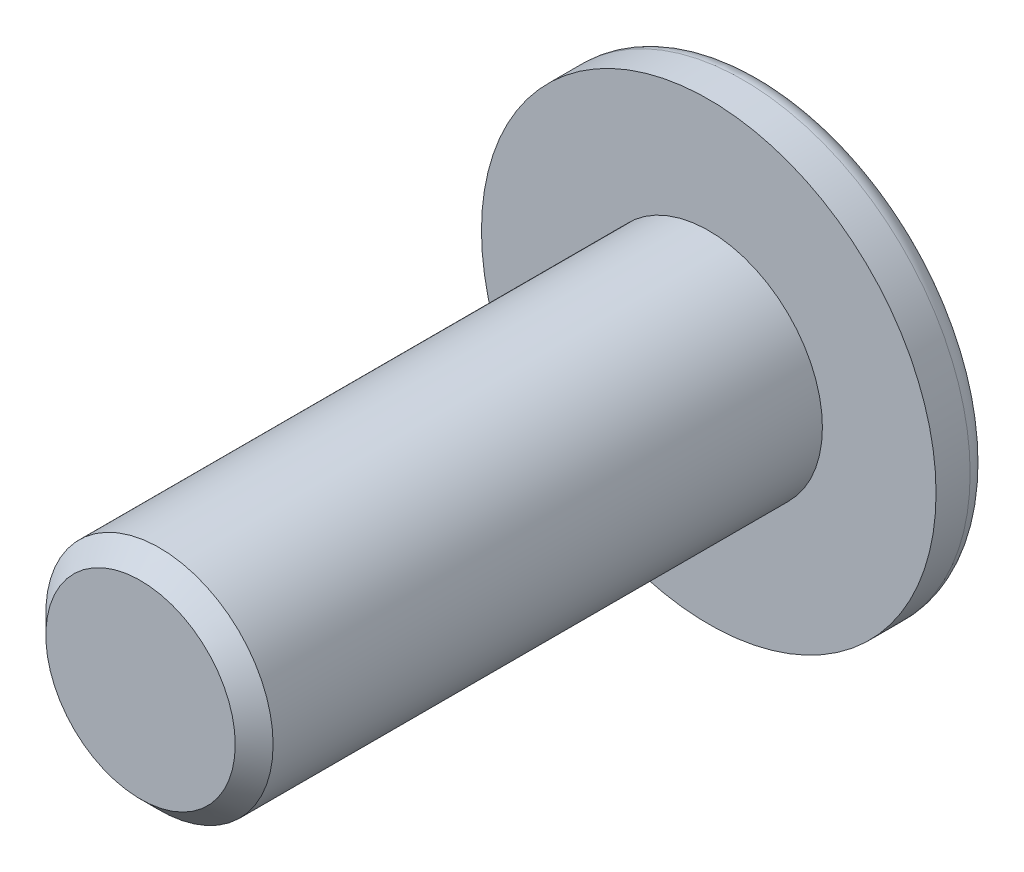
from build123d import *

# Parameters (mm, degrees)
SKETCH_1_R          = 6
EXTRUDE_1_DEPTH     = 1.4
SKETCH_2_R          = 3
EXTRUDE_2_DEPTH     = 15
FILLET_1_R          = 0.5
CUT_EXTRUDE_1_DEPTH = 2
CHAMFER_1_SIZE      = 0.5


with BuildPart() as part:
    # 草图1 → 凸台-拉伸1 (new body)
    with BuildSketch(Plane.XY):
        Circle(SKETCH_1_R)
    extrude(amount=EXTRUDE_1_DEPTH)

    # 草图2 → 凸台-拉伸2 (add)
    with BuildSketch(Plane.XY.offset(1.4)):
        Circle(SKETCH_2_R)
    extrude(amount=EXTRUDE_2_DEPTH)

    # 圆角1
    fillet_1_edges = [part.edges().sort_by_distance(p)[0] for p in [
        (-6, 0, 0),
    ]]
    fillet(fillet_1_edges, radius=FILLET_1_R)

    # 草图3 → 切除-拉伸1 (cut)
    with BuildSketch(Plane(origin=(0, 0, 0), x_dir=(-1, 0, 0), z_dir=(0, 0, -1))):
        Polygon((0.749542431, -2.184380799), (2.266500479, -0.443067613), (1.516958048, 1.741313186), (-0.749542431, 2.184380799), (-2.266500479, 0.443067613), (-1.516958048, -1.741313186), align=None)
    extrude(amount=-CUT_EXTRUDE_1_DEPTH, mode=Mode.SUBTRACT)

    # 倒角1
    chamfer_1_edges = [part.edges().sort_by_distance(p)[0] for p in [
        (-3, 0, 16.4),
    ]]
    chamfer(chamfer_1_edges, length=CHAMFER_1_SIZE)


solid = part.part
